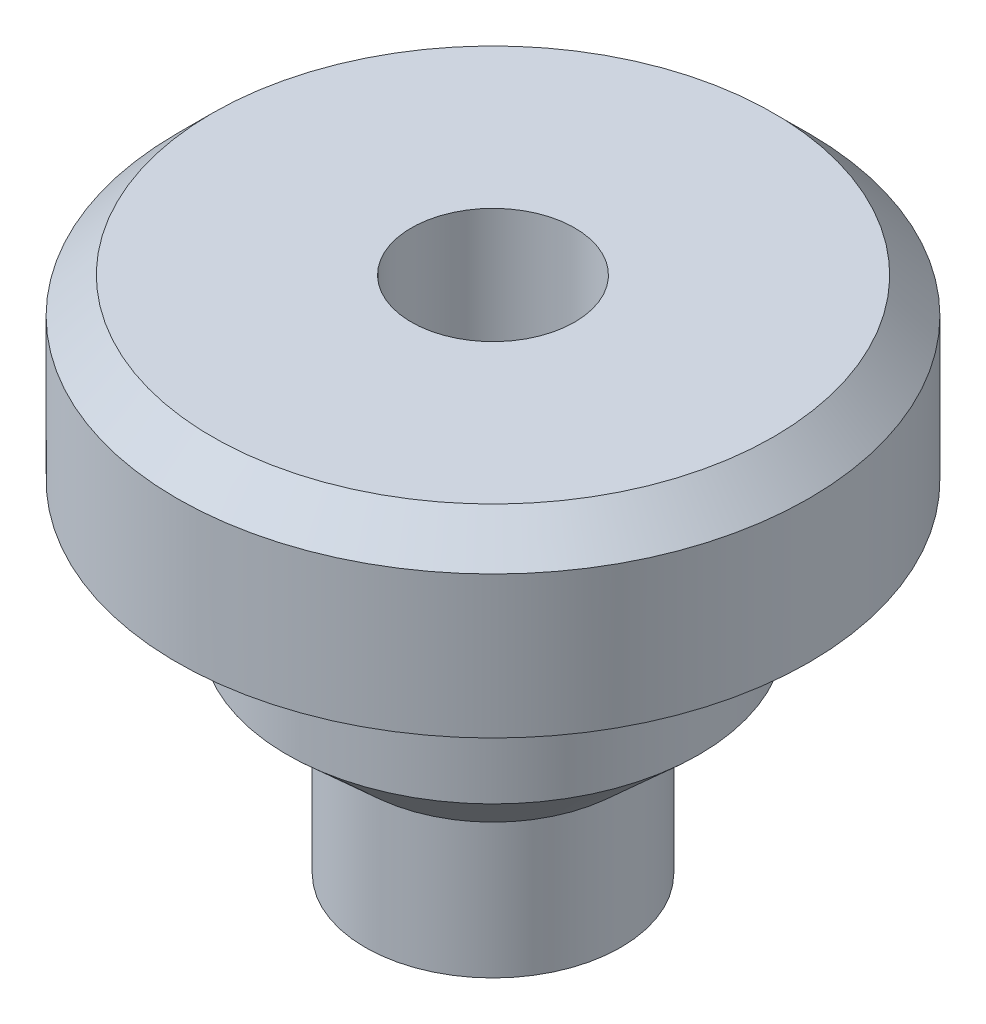
SolidWorks part; units mm, degrees
material "Rubber"
ref_plane "Front Plane" through (0, 0, 0) normal (0, 0, 1) x (1, 0, 0)
ref_plane "Top Plane" through (0, 0, 0) normal (0, 1, 0) x (1, 0, 0)
ref_plane "Right Plane" through (0, 0, 0) normal (1, 0, 0) x (0, 0, -1)
sketch "Sketch1" plane through (0, 0, 0) normal (0, 0, 1) x (1, 0, 0)
  line L0 (0, -693.7992) -> (0, 33996.1614) construction
  line L1 (11.5, 0) -> (11.5, 73)
  line L2 (11.5, 73) -> (44.5, 73)
  line L3 (44.5, 73) -> (44.5, 48)
  line L4 (44.5, 48) -> (29, 48)
  line L5 (29, 48) -> (29, 29)
  line L6 (29, 29) -> (18, 19)
  line L7 (18, 19) -> (18, 0)
  line L8 (18, 0) -> (11.5, 0)
  dimension "D1" = 11.5
  dimension "D2" = 44.5
  dimension "D3" = 29
  dimension "D4" = 73
  dimension "D5" = 25
  dimension "D6" = 19
  dimension "D7" = 18
  dimension "D8" = 10
revolve "Revolve1" add sketch "Sketch1" angle 360 about L0
chamfer "Chamfer1" distance 5 angle 45 1 edges at (44.5, 73, 0)
